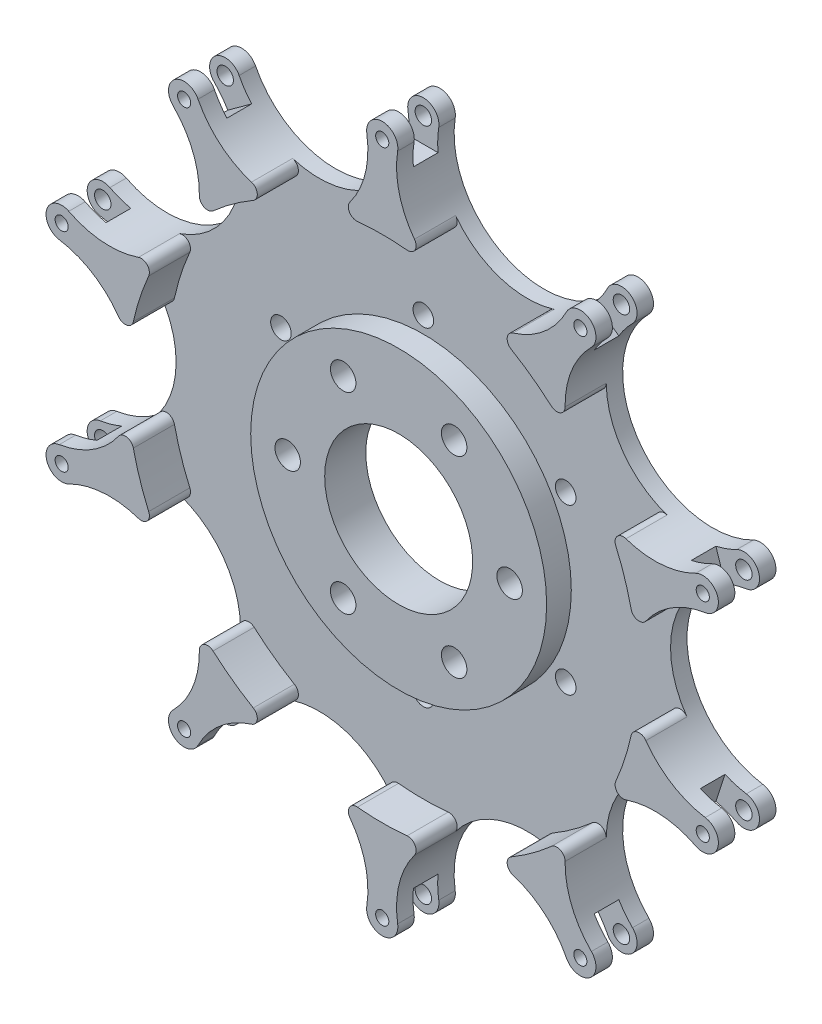
from build123d import *
from build123d.topology import SkipClean

# Parameters (mm, degrees)
SKETCH_1_R             = 1
EXTRUDE_1031_DEPTH     = 2
HOLE_WIZARD_M3_1_D     = 2.5
CUT_EXTRUDE_4270_REACH = 61.302
SKETCH_7_R             = 1.55
SKETCH_7_R_2           = 9
SKETCH_12_R            = 18
SKETCH_12_R_2          = 1.55
SKETCH_12_R_3          = 9
EXTRUDE_1_DEPTH        = 3
EXTRUDE_2_DEPTH        = 3
EXTRUDE_3_DEPTH        = 2
HOLE_WIZARD_M2_1_D     = 1.6


with BuildPart() as part:
    # 草图1 → Extrude 1031 (new body)
    with BuildSketch(Plane.XY):
        with BuildLine():
            ThreePointArc((1.876607847, 40.702774516), (0, 42.9), (-1.876607847, 40.702774516))
            ThreePointArc((-1.876607847, 40.702774516), (-3.352363827, 33.283648198), (-9.292874586, 28.600527126))
            ThreePointArc((-9.292874586, 28.600527126), (-16.851518246, 28.897507045), (-22.406282948, 34.032278719))
            ThreePointArc((-22.406282948, 34.032278719), (-25.215987323, 34.706829059), (-25.442698228, 31.826193885))
            ThreePointArc((-25.442698228, 31.826193885), (-22.275756861, 24.956567009), (-24.329061519, 17.67609786))
            ThreePointArc((-24.329061519, 17.67609786), (-30.618693111, 13.473500391), (-38.130735219, 14.362609165))
            ThreePointArc((-38.130735219, 14.362609165), (-40.800324549, 13.256829059), (-39.290542652, 10.793088922))
            ThreePointArc((-39.290542652, 10.793088922), (-32.690567898, 7.096925465), (-30.072373867, 0))
            ThreePointArc((-30.072373867, 0), (-32.690567898, -7.096925465), (-39.290542652, -10.793088922))
            ThreePointArc((-39.290542652, -10.793088922), (-40.800324549, -13.256829059), (-38.130735219, -14.362609165))
            ThreePointArc((-38.130735219, -14.362609165), (-30.618693111, -13.473500391), (-24.329061519, -17.67609786))
            ThreePointArc((-24.329061519, -17.67609786), (-22.275756861, -24.956567009), (-25.442698228, -31.826193885))
            ThreePointArc((-25.442698228, -31.826193885), (-25.215987323, -34.706829059), (-22.406282948, -34.032278719))
            ThreePointArc((-22.406282948, -34.032278719), (-16.851518246, -28.897507045), (-9.292874586, -28.600527126))
            ThreePointArc((-9.292874586, -28.600527126), (-3.352363827, -33.283648198), (-1.876607847, -40.702774516))
            ThreePointArc((-1.876607847, -40.702774516), (0, -42.9), (1.876607847, -40.702774516))
            ThreePointArc((1.876607847, -40.702774516), (3.352363827, -33.283648198), (9.292874586, -28.600527126))
            ThreePointArc((9.292874586, -28.600527126), (16.851518246, -28.897507045), (22.406282948, -34.032278719))
            ThreePointArc((22.406282948, -34.032278719), (25.215987323, -34.706829059), (25.442698228, -31.826193885))
            ThreePointArc((25.442698228, -31.826193885), (22.275756861, -24.956567009), (24.329061519, -17.67609786))
            ThreePointArc((24.329061519, -17.67609786), (30.618693111, -13.473500391), (38.130735219, -14.362609165))
            ThreePointArc((38.130735219, -14.362609165), (40.800324549, -13.256829059), (39.290542652, -10.793088922))
            ThreePointArc((39.290542652, -10.793088922), (32.690567898, -7.096925465), (30.072373867, 0))
            ThreePointArc((30.072373867, 0), (32.690567898, 7.096925465), (39.290542652, 10.793088922))
            ThreePointArc((39.290542652, 10.793088922), (40.800324549, 13.256829059), (38.130735219, 14.362609165))
            ThreePointArc((38.130735219, 14.362609165), (30.618693111, 13.473500391), (24.329061519, 17.67609786))
            ThreePointArc((24.329061519, 17.67609786), (22.275756861, 24.956567009), (25.442698228, 31.826193885))
            ThreePointArc((25.442698228, 31.826193885), (25.215987323, 34.706829059), (22.406282948, 34.032278719))
            ThreePointArc((22.406282948, 34.032278719), (16.851518246, 28.897507045), (9.292874586, 28.600527126))
            ThreePointArc((9.292874586, 28.600527126), (3.352363827, 33.283648198), (1.876607847, 40.702774516))
        make_face()
        with Locations((0, 41)):
            Circle(SKETCH_1_R, mode=Mode.SUBTRACT)
        with Locations((24.099195344, 33.169696769)):
            Circle(SKETCH_1_R, mode=Mode.SUBTRACT)
        with Locations((38.993317168, 12.669696769)):
            Circle(SKETCH_1_R, mode=Mode.SUBTRACT)
        with Locations((38.993317168, -12.669696769)):
            Circle(SKETCH_1_R, mode=Mode.SUBTRACT)
        with Locations((24.099195344, -33.169696769)):
            Circle(SKETCH_1_R, mode=Mode.SUBTRACT)
        with Locations((0, -41)):
            Circle(SKETCH_1_R, mode=Mode.SUBTRACT)
        with Locations((-24.099195344, -33.169696769)):
            Circle(SKETCH_1_R, mode=Mode.SUBTRACT)
        with Locations((-38.993317168, -12.669696769)):
            Circle(SKETCH_1_R, mode=Mode.SUBTRACT)
        with Locations((-38.993317168, 12.669696769)):
            Circle(SKETCH_1_R, mode=Mode.SUBTRACT)
        with Locations((-24.099195344, 33.169696769)):
            Circle(SKETCH_1_R, mode=Mode.SUBTRACT)
    extrude(amount=EXTRUDE_1031_DEPTH)

    # M3 螺纹孔1 (through all)
    with Locations(Plane(origin=(0, 0, 0), x_dir=(-1, 0, 0), z_dir=(0, 0, -1))):
        with Locations((-17.320508076, 10), (0, 20), (17.320508076, 10), (17.320508076, -10), (0, -20), (-17.320508076, -10), (0, 0)):
            Hole(HOLE_WIZARD_M3_1_D / 2)

    # 草图7 → Cut-Extrude 4270 (cut, up to next)
    with BuildSketch(Plane(origin=(0, 0, 0), x_dir=(-1, 0, 0), z_dir=(0, 0, -1)), mode=Mode.PRIVATE) as cut_extrude_4270_sk1:
        with Locations((13.5, 0)):
            Circle(SKETCH_7_R)
    cut_extrude_4270_tool1 = extrude(cut_extrude_4270_sk1.sketch, amount=-CUT_EXTRUDE_4270_REACH, mode=Mode.PRIVATE) & part.part
    # 草图7 → Cut-Extrude 4270 (cut, up to next)
    with BuildSketch(Plane(origin=(0, 0, 0), x_dir=(-1, 0, 0), z_dir=(0, 0, -1)), mode=Mode.PRIVATE) as cut_extrude_4270_sk2:
        with Locations((6.75, -11.691342951)):
            Circle(SKETCH_7_R)
    cut_extrude_4270_tool2 = extrude(cut_extrude_4270_sk2.sketch, amount=-CUT_EXTRUDE_4270_REACH, mode=Mode.PRIVATE) & part.part
    # 草图7 → Cut-Extrude 4270 (cut, up to next)
    with BuildSketch(Plane(origin=(0, 0, 0), x_dir=(-1, 0, 0), z_dir=(0, 0, -1)), mode=Mode.PRIVATE) as cut_extrude_4270_sk3:
        with Locations((-6.75, -11.691342951)):
            Circle(SKETCH_7_R)
    cut_extrude_4270_tool3 = extrude(cut_extrude_4270_sk3.sketch, amount=-CUT_EXTRUDE_4270_REACH, mode=Mode.PRIVATE) & part.part
    # 草图7 → Cut-Extrude 4270 (cut, up to next)
    with BuildSketch(Plane(origin=(0, 0, 0), x_dir=(-1, 0, 0), z_dir=(0, 0, -1)), mode=Mode.PRIVATE) as cut_extrude_4270_sk4:
        with Locations((-13.5, 0)):
            Circle(SKETCH_7_R)
    cut_extrude_4270_tool4 = extrude(cut_extrude_4270_sk4.sketch, amount=-CUT_EXTRUDE_4270_REACH, mode=Mode.PRIVATE) & part.part
    # 草图7 → Cut-Extrude 4270 (cut, up to next)
    with BuildSketch(Plane(origin=(0, 0, 0), x_dir=(-1, 0, 0), z_dir=(0, 0, -1)), mode=Mode.PRIVATE) as cut_extrude_4270_sk5:
        with Locations((-6.75, 11.691342951)):
            Circle(SKETCH_7_R)
    cut_extrude_4270_tool5 = extrude(cut_extrude_4270_sk5.sketch, amount=-CUT_EXTRUDE_4270_REACH, mode=Mode.PRIVATE) & part.part
    # 草图7 → Cut-Extrude 4270 (cut, up to next)
    with BuildSketch(Plane(origin=(0, 0, 0), x_dir=(-1, 0, 0), z_dir=(0, 0, -1)), mode=Mode.PRIVATE) as cut_extrude_4270_sk6:
        with Locations((6.75, 11.691342951)):
            Circle(SKETCH_7_R)
    cut_extrude_4270_tool6 = extrude(cut_extrude_4270_sk6.sketch, amount=-CUT_EXTRUDE_4270_REACH, mode=Mode.PRIVATE) & part.part
    # 草图7 → Cut-Extrude 4270 (cut, up to next)
    with BuildSketch(Plane(origin=(0, 0, 0), x_dir=(-1, 0, 0), z_dir=(0, 0, -1)), mode=Mode.PRIVATE) as cut_extrude_4270_sk7:
        Circle(SKETCH_7_R_2)
    cut_extrude_4270_tool7 = extrude(cut_extrude_4270_sk7.sketch, amount=-CUT_EXTRUDE_4270_REACH, mode=Mode.PRIVATE) & part.part
    add(cut_extrude_4270_tool1.solids().sort_by_distance((-13.5, 0, 0))[0], mode=Mode.SUBTRACT)
    add(cut_extrude_4270_tool2.solids().sort_by_distance((-6.75, -11.691343, 0))[0], mode=Mode.SUBTRACT)
    add(cut_extrude_4270_tool3.solids().sort_by_distance((6.75, -11.691343, 0))[0], mode=Mode.SUBTRACT)
    add(cut_extrude_4270_tool4.solids().sort_by_distance((13.5, 0, 0))[0], mode=Mode.SUBTRACT)
    add(cut_extrude_4270_tool5.solids().sort_by_distance((6.75, 11.691343, 0))[0], mode=Mode.SUBTRACT)
    add(cut_extrude_4270_tool6.solids().sort_by_distance((-6.75, 11.691343, 0))[0], mode=Mode.SUBTRACT)
    add(cut_extrude_4270_tool7.solids().sort_by_distance((0, 0, 0))[0], mode=Mode.SUBTRACT)

    # 草图12 → 凸台-拉伸1 (add)
    with BuildSketch(Plane(origin=(0, 0, 2), x_dir=(-1, 0, 0), z_dir=(0, 0, -1))):
        Circle(SKETCH_12_R)
        with Locations((6.75, 11.691342951)):
            Circle(SKETCH_12_R_2, mode=Mode.SUBTRACT)
        with Locations((13.5, 0)):
            Circle(SKETCH_12_R_2, mode=Mode.SUBTRACT)
        with Locations((6.75, -11.691342951)):
            Circle(SKETCH_12_R_2, mode=Mode.SUBTRACT)
        with Locations((-6.75, -11.691342951)):
            Circle(SKETCH_12_R_2, mode=Mode.SUBTRACT)
        with Locations((-13.5, 0)):
            Circle(SKETCH_12_R_2, mode=Mode.SUBTRACT)
        with Locations((-6.75, 11.691342951)):
            Circle(SKETCH_12_R_2, mode=Mode.SUBTRACT)
        Circle(SKETCH_12_R_3, mode=Mode.SUBTRACT)
    extrude(amount=-EXTRUDE_1_DEPTH)

    # 草图13 → 凸台-拉伸2 (add)
    with SkipClean():  # the faces are left unmerged after this step: merging them gives an invalid solid
        with BuildSketch(Plane.XY.offset(2)):
            with BuildLine():
                Line((-1.787310362, 38), (1.787310362, 38))
                ThreePointArc((1.787310362, 38), (2.468567924, 35.075411709), (3.920151332, 32.446679287))
                ThreePointArc((3.920151332, 32.446679287), (3.990728944, 31.356764929), (3.021986634, 30.85235156))
                ThreePointArc((3.021986634, 30.85235156), (0, 31), (-3.021986634, 30.85235156))
                ThreePointArc((-3.021986634, 30.85235156), (-3.990728944, 31.356764929), (-3.920151332, 32.446679287))
                ThreePointArc((-3.920151332, 32.446679287), (-2.468567924, 35.075411709), (-1.787310362, 38))
            make_face()
            with BuildLine():
                Line((20.88987513, 31.793200458), (23.781804044, 29.692091114))
                ThreePointArc((23.781804044, 29.692091114), (22.613923123, 26.925616338), (22.243148619, 23.945707815))
                ThreePointArc((22.243148619, 23.945707815), (21.65961152, 23.022464097), (20.579395789, 23.183797552))
                ThreePointArc((20.579395789, 23.183797552), (18.221342821, 25.079526826), (15.689718702, 26.736355905))
                ThreePointArc((15.689718702, 26.736355905), (15.202476449, 27.713847335), (15.900210523, 28.554122094))
                ThreePointArc((15.900210523, 28.554122094), (18.619696319, 29.827591977), (20.88987513, 31.793200458))
            make_face()
            with BuildLine():
                Line((35.587838343, 13.442478953), (36.692456895, 10.04281262))
                ThreePointArc((36.692456895, 10.04281262), (34.121528308, 8.491150693), (32.07001915, 6.298289842))
                ThreePointArc((32.07001915, 6.298289842), (31.055258679, 5.894364485), (30.276175221, 6.659820868))
                ThreePointArc((30.276175221, 6.659820868), (29.482752005, 9.579526826), (28.408484768, 12.407981029))
                ThreePointArc((28.408484768, 12.407981029), (28.588852552, 13.485182018), (29.647232386, 13.75486078))
                ThreePointArc((29.647232386, 13.75486078), (32.595869428, 13.186645913), (35.587838343, 13.442478953))
            make_face()
            with BuildLine():
                Line((36.692456895, -10.04281262), (35.587838343, -13.442478953))
                ThreePointArc((35.587838343, -13.442478953), (32.595869428, -13.186645913), (29.647232386, -13.75486078))
                ThreePointArc((29.647232386, -13.75486078), (28.588852552, -13.485182018), (28.408484768, -12.407981029))
                ThreePointArc((28.408484768, -12.407981029), (29.482752005, -9.579526826), (30.276175221, -6.659820868))
                ThreePointArc((30.276175221, -6.659820868), (31.055258679, -5.894364485), (32.07001915, -6.298289842))
                ThreePointArc((32.07001915, -6.298289842), (34.121528308, -8.491150693), (36.692456895, -10.04281262))
            make_face()
            with BuildLine():
                Line((23.781804044, -29.692091114), (20.88987513, -31.793200458))
                ThreePointArc((20.88987513, -31.793200458), (18.619696319, -29.827591977), (15.900210523, -28.554122094))
                ThreePointArc((15.900210523, -28.554122094), (15.202476449, -27.713847335), (15.689718702, -26.736355905))
                ThreePointArc((15.689718702, -26.736355905), (18.221342821, -25.079526826), (20.579395789, -23.183797552))
                ThreePointArc((20.579395789, -23.183797552), (21.65961152, -23.022464097), (22.243148619, -23.945707815))
                ThreePointArc((22.243148619, -23.945707815), (22.613923123, -26.925616338), (23.781804044, -29.692091114))
            make_face()
            with BuildLine():
                Line((1.787310362, -38), (-1.787310362, -38))
                ThreePointArc((-1.787310362, -38), (-2.468567924, -35.075411709), (-3.920151332, -32.446679287))
                ThreePointArc((-3.920151332, -32.446679287), (-3.990728944, -31.356764929), (-3.021986634, -30.85235156))
                ThreePointArc((-3.021986634, -30.85235156), (0, -31), (3.021986634, -30.85235156))
                ThreePointArc((3.021986634, -30.85235156), (3.990728944, -31.356764929), (3.920151332, -32.446679287))
                ThreePointArc((3.920151332, -32.446679287), (2.468567924, -35.075411709), (1.787310362, -38))
            make_face()
            with BuildLine():
                Line((-20.88987513, -31.793200458), (-23.781804044, -29.692091114))
                ThreePointArc((-23.781804044, -29.692091114), (-22.613923123, -26.925616338), (-22.243148619, -23.945707815))
                ThreePointArc((-22.243148619, -23.945707815), (-21.65961152, -23.022464097), (-20.579395789, -23.183797552))
                ThreePointArc((-20.579395789, -23.183797552), (-18.221342821, -25.079526826), (-15.689718702, -26.736355905))
                ThreePointArc((-15.689718702, -26.736355905), (-15.202476449, -27.713847335), (-15.900210523, -28.554122094))
                ThreePointArc((-15.900210523, -28.554122094), (-18.619696319, -29.827591977), (-20.88987513, -31.793200458))
            make_face()
            with BuildLine():
                Line((-35.587838343, -13.442478953), (-36.692456895, -10.04281262))
                ThreePointArc((-36.692456895, -10.04281262), (-34.121528308, -8.491150693), (-32.07001915, -6.298289842))
                ThreePointArc((-32.07001915, -6.298289842), (-31.055258679, -5.894364485), (-30.276175221, -6.659820868))
                ThreePointArc((-30.276175221, -6.659820868), (-29.482752005, -9.579526826), (-28.408484768, -12.407981029))
                ThreePointArc((-28.408484768, -12.407981029), (-28.588852552, -13.485182018), (-29.647232386, -13.75486078))
                ThreePointArc((-29.647232386, -13.75486078), (-32.595869428, -13.186645913), (-35.587838343, -13.442478953))
            make_face()
            with BuildLine():
                Line((-36.692456895, 10.04281262), (-35.587838343, 13.442478953))
                ThreePointArc((-35.587838343, 13.442478953), (-32.595869428, 13.186645913), (-29.647232386, 13.75486078))
                ThreePointArc((-29.647232386, 13.75486078), (-28.588852552, 13.485182018), (-28.408484768, 12.407981029))
                ThreePointArc((-28.408484768, 12.407981029), (-29.482752005, 9.579526826), (-30.276175221, 6.659820868))
                ThreePointArc((-30.276175221, 6.659820868), (-31.055258679, 5.894364485), (-32.07001915, 6.298289842))
                ThreePointArc((-32.07001915, 6.298289842), (-34.121528308, 8.491150693), (-36.692456895, 10.04281262))
            make_face()
            with BuildLine():
                Line((-23.781804044, 29.692091114), (-20.88987513, 31.793200458))
                ThreePointArc((-20.88987513, 31.793200458), (-18.619696319, 29.827591977), (-15.900210523, 28.554122094))
                ThreePointArc((-15.900210523, 28.554122094), (-15.202476449, 27.713847335), (-15.689718702, 26.736355905))
                ThreePointArc((-15.689718702, 26.736355905), (-18.221342821, 25.079526826), (-20.579395789, 23.183797552))
                ThreePointArc((-20.579395789, 23.183797552), (-21.65961152, 23.022464097), (-22.243148619, 23.945707815))
                ThreePointArc((-22.243148619, 23.945707815), (-22.613923123, 26.925616338), (-23.781804044, 29.692091114))
            make_face()
        extrude(amount=EXTRUDE_2_DEPTH)

    # 草图14 → 凸台-拉伸3 (add)
    with SkipClean():  # the faces are left unmerged after this step: merging them gives an invalid solid
        with BuildSketch(Plane.XY.offset(5)):
            with BuildLine():
                ThreePointArc((1.876607847, 40.702774516), (1.748029991, 39.354160208), (1.787310362, 38))
                ThreePointArc((1.787310362, 38), (2.468567924, 35.075411709), (3.920151332, 32.446679287))
                ThreePointArc((3.920151332, 32.446679287), (3.990728944, 31.356764929), (3.021986634, 30.85235156))
                ThreePointArc((3.021986634, 30.85235156), (0, 31), (-3.021986634, 30.85235156))
                ThreePointArc((-3.021986634, 30.85235156), (-3.990728944, 31.356764929), (-3.920151332, 32.446679287))
                ThreePointArc((-3.920151332, 32.446679287), (-2.468567924, 35.075411709), (-1.787310362, 38))
                ThreePointArc((-1.787310362, 38), (-1.748029991, 39.354160208), (-1.876607847, 40.702774516))
                ThreePointArc((-1.876607847, 40.702774516), (0, 42.9), (1.876607847, 40.702774516))
            make_face()
            with BuildLine():
                ThreePointArc((20.88987513, 31.793200458), (21.717609017, 32.865650657), (22.406282948, 34.032278719))
                ThreePointArc((22.406282948, 34.032278719), (25.215987323, 34.706829059), (25.442698228, 31.826193885))
                ThreePointArc((25.442698228, 31.826193885), (24.545980956, 30.810718158), (23.781804044, 29.692091114))
                ThreePointArc((23.781804044, 29.692091114), (22.613923123, 26.925616338), (22.243148619, 23.945707815))
                ThreePointArc((22.243148619, 23.945707815), (21.65961152, 23.022464097), (20.579395789, 23.183797552))
                ThreePointArc((20.579395789, 23.183797552), (18.221342821, 25.079526826), (15.689718702, 26.736355905))
                ThreePointArc((15.689718702, 26.736355905), (15.202476449, 27.713847335), (15.900210523, 28.554122094))
                ThreePointArc((15.900210523, 28.554122094), (18.619696319, 29.827591977), (20.88987513, 31.793200458))
            make_face()
            with BuildLine():
                ThreePointArc((35.587838343, 13.442478953), (36.887859535, 13.823579618), (38.130735219, 14.362609165))
                ThreePointArc((38.130735219, 14.362609165), (40.800324549, 13.256829059), (39.290542652, 10.793088922))
                ThreePointArc((39.290542652, 10.793088922), (37.968201483, 10.49862899), (36.692456895, 10.04281262))
                ThreePointArc((36.692456895, 10.04281262), (34.121528308, 8.491150693), (32.07001915, 6.298289842))
                ThreePointArc((32.07001915, 6.298289842), (31.055258679, 5.894364485), (30.276175221, 6.659820868))
                ThreePointArc((30.276175221, 6.659820868), (29.482752005, 9.579526826), (28.408484768, 12.407981029))
                ThreePointArc((28.408484768, 12.407981029), (28.588852552, 13.485182018), (29.647232386, 13.75486078))
                ThreePointArc((29.647232386, 13.75486078), (32.595869428, 13.186645913), (35.587838343, 13.442478953))
            make_face()
            with BuildLine():
                ThreePointArc((36.692456895, -10.04281262), (37.968201483, -10.49862899), (39.290542652, -10.793088922))
                ThreePointArc((39.290542652, -10.793088922), (40.800324549, -13.256829059), (38.130735219, -14.362609165))
                ThreePointArc((38.130735219, -14.362609165), (36.887859535, -13.823579618), (35.587838343, -13.442478953))
                ThreePointArc((35.587838343, -13.442478953), (32.595869428, -13.186645913), (29.647232386, -13.75486078))
                ThreePointArc((29.647232386, -13.75486078), (28.588852552, -13.485182018), (28.408484768, -12.407981029))
                ThreePointArc((28.408484768, -12.407981029), (29.482752005, -9.579526826), (30.276175221, -6.659820868))
                ThreePointArc((30.276175221, -6.659820868), (31.055258679, -5.894364485), (32.07001915, -6.298289842))
                ThreePointArc((32.07001915, -6.298289842), (34.121528308, -8.491150693), (36.692456895, -10.04281262))
            make_face()
            with BuildLine():
                ThreePointArc((23.781804044, -29.692091114), (24.545980956, -30.810718158), (25.442698228, -31.826193885))
                ThreePointArc((25.442698228, -31.826193885), (25.215987323, -34.706829059), (22.406282948, -34.032278719))
                ThreePointArc((22.406282948, -34.032278719), (21.717609017, -32.865650657), (20.88987513, -31.793200458))
                ThreePointArc((20.88987513, -31.793200458), (18.619696319, -29.827591977), (15.900210523, -28.554122094))
                ThreePointArc((15.900210523, -28.554122094), (15.202476449, -27.713847335), (15.689718702, -26.736355905))
                ThreePointArc((15.689718702, -26.736355905), (18.221342821, -25.079526826), (20.579395789, -23.183797552))
                ThreePointArc((20.579395789, -23.183797552), (21.65961152, -23.022464097), (22.243148619, -23.945707815))
                ThreePointArc((22.243148619, -23.945707815), (22.613923123, -26.925616338), (23.781804044, -29.692091114))
            make_face()
            with BuildLine():
                ThreePointArc((1.787310362, -38), (1.748029991, -39.354160208), (1.876607847, -40.702774516))
                ThreePointArc((1.876607847, -40.702774516), (0, -42.9), (-1.876607847, -40.702774516))
                ThreePointArc((-1.876607847, -40.702774516), (-1.748029991, -39.354160208), (-1.787310362, -38))
                ThreePointArc((-1.787310362, -38), (-2.468567924, -35.075411709), (-3.920151332, -32.446679287))
                ThreePointArc((-3.920151332, -32.446679287), (-3.990728944, -31.356764929), (-3.021986634, -30.85235156))
                ThreePointArc((-3.021986634, -30.85235156), (0, -31), (3.021986634, -30.85235156))
                ThreePointArc((3.021986634, -30.85235156), (3.990728944, -31.356764929), (3.920151332, -32.446679287))
                ThreePointArc((3.920151332, -32.446679287), (2.468567924, -35.075411709), (1.787310362, -38))
            make_face()
            with BuildLine():
                ThreePointArc((-20.88987513, -31.793200458), (-21.717609017, -32.865650657), (-22.406282948, -34.032278719))
                ThreePointArc((-22.406282948, -34.032278719), (-25.215987323, -34.706829059), (-25.442698228, -31.826193885))
                ThreePointArc((-25.442698228, -31.826193885), (-24.545980956, -30.810718158), (-23.781804044, -29.692091114))
                ThreePointArc((-23.781804044, -29.692091114), (-22.613923123, -26.925616338), (-22.243148619, -23.945707815))
                ThreePointArc((-22.243148619, -23.945707815), (-21.65961152, -23.022464097), (-20.579395789, -23.183797552))
                ThreePointArc((-20.579395789, -23.183797552), (-18.221342821, -25.079526826), (-15.689718702, -26.736355905))
                ThreePointArc((-15.689718702, -26.736355905), (-15.202476449, -27.713847335), (-15.900210523, -28.554122094))
                ThreePointArc((-15.900210523, -28.554122094), (-18.619696319, -29.827591977), (-20.88987513, -31.793200458))
            make_face()
            with BuildLine():
                ThreePointArc((-35.587838343, -13.442478953), (-36.887859535, -13.823579618), (-38.130735219, -14.362609165))
                ThreePointArc((-38.130735219, -14.362609165), (-40.800324549, -13.256829059), (-39.290542652, -10.793088922))
                ThreePointArc((-39.290542652, -10.793088922), (-37.968201483, -10.49862899), (-36.692456895, -10.04281262))
                ThreePointArc((-36.692456895, -10.04281262), (-34.121528308, -8.491150693), (-32.07001915, -6.298289842))
                ThreePointArc((-32.07001915, -6.298289842), (-31.055258679, -5.894364485), (-30.276175221, -6.659820868))
                ThreePointArc((-30.276175221, -6.659820868), (-29.482752005, -9.579526826), (-28.408484768, -12.407981029))
                ThreePointArc((-28.408484768, -12.407981029), (-28.588852552, -13.485182018), (-29.647232386, -13.75486078))
                ThreePointArc((-29.647232386, -13.75486078), (-32.595869428, -13.186645913), (-35.587838343, -13.442478953))
            make_face()
            with BuildLine():
                ThreePointArc((-36.692456895, 10.04281262), (-37.968201483, 10.49862899), (-39.290542652, 10.793088922))
                ThreePointArc((-39.290542652, 10.793088922), (-40.800324549, 13.256829059), (-38.130735219, 14.362609165))
                ThreePointArc((-38.130735219, 14.362609165), (-36.887859535, 13.823579618), (-35.587838343, 13.442478953))
                ThreePointArc((-35.587838343, 13.442478953), (-32.595869428, 13.186645913), (-29.647232386, 13.75486078))
                ThreePointArc((-29.647232386, 13.75486078), (-28.588852552, 13.485182018), (-28.408484768, 12.407981029))
                ThreePointArc((-28.408484768, 12.407981029), (-29.482752005, 9.579526826), (-30.276175221, 6.659820868))
                ThreePointArc((-30.276175221, 6.659820868), (-31.055258679, 5.894364485), (-32.07001915, 6.298289842))
                ThreePointArc((-32.07001915, 6.298289842), (-34.121528308, 8.491150693), (-36.692456895, 10.04281262))
            make_face()
            with BuildLine():
                ThreePointArc((-23.781804044, 29.692091114), (-24.545980956, 30.810718158), (-25.442698228, 31.826193885))
                ThreePointArc((-25.442698228, 31.826193885), (-25.215987323, 34.706829059), (-22.406282948, 34.032278719))
                ThreePointArc((-22.406282948, 34.032278719), (-21.717609017, 32.865650657), (-20.88987513, 31.793200458))
                ThreePointArc((-20.88987513, 31.793200458), (-18.619696319, 29.827591977), (-15.900210523, 28.554122094))
                ThreePointArc((-15.900210523, 28.554122094), (-15.202476449, 27.713847335), (-15.689718702, 26.736355905))
                ThreePointArc((-15.689718702, 26.736355905), (-18.221342821, 25.079526826), (-20.579395789, 23.183797552))
                ThreePointArc((-20.579395789, 23.183797552), (-21.65961152, 23.022464097), (-22.243148619, 23.945707815))
                ThreePointArc((-22.243148619, 23.945707815), (-22.613923123, 26.925616338), (-23.781804044, 29.692091114))
            make_face()
        extrude(amount=EXTRUDE_3_DEPTH)

    # M2 螺纹孔1 (through all)
    with Locations(Plane.XY.offset(7)):
        with Locations((0, 41), (24.099195344, 33.169696769), (38.993317168, 12.669696769), (38.993317168, -12.669696769), (24.099195344, -33.169696769), (0, -41), (-24.099195344, -33.169696769), (-38.993317168, -12.669696769), (-38.993317168, 12.669696769), (-24.099195344, 33.169696769), (0, 0)):
            Hole(HOLE_WIZARD_M2_1_D / 2)


solid = part.part
